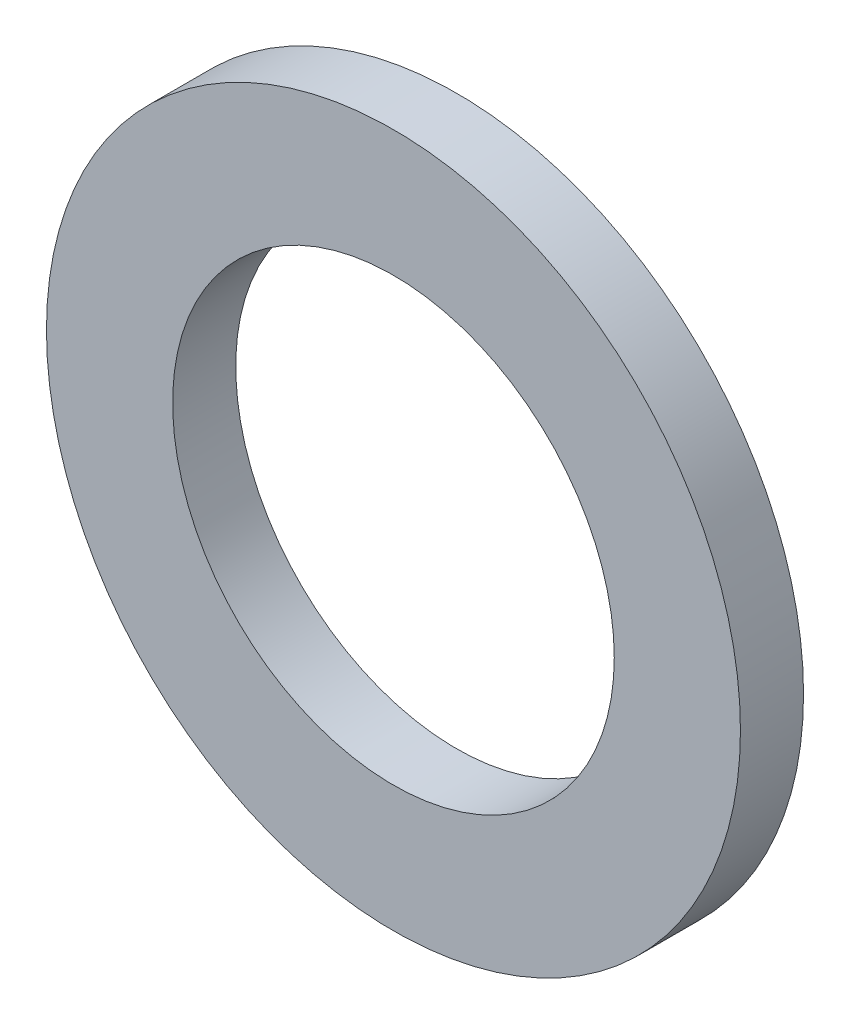
SolidWorks part; units mm, degrees
ref_plane "Front Plane" through (0, 0, 0) normal (0, 0, 1) x (1, 0, 0)
ref_plane "Top Plane" through (0, 0, 0) normal (0, 1, 0) x (1, 0, 0)
ref_plane "Right Plane" through (0, 0, 0) normal (1, 0, 0) x (0, 0, -1)
other "Configuration Table"
sketch "Sketch1" plane through (0, 0, 0) normal (0, 0, 1) x (1, 0, 0)
  circle A0 centre (0, 0) radius 11
  circle A1 centre (0, 0) radius 7
  dimension "D1" = 22
  dimension "D2" = 14
extrude "Boss-Extrude1" add sketch "Sketch1" along normal blind 2
